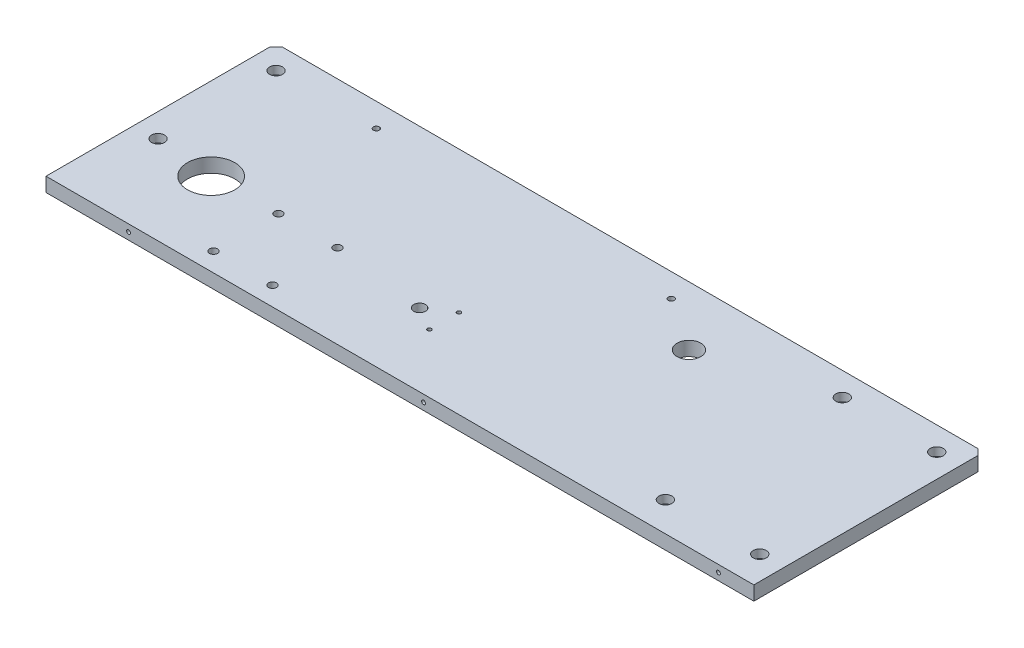
from build123d import *

# Parameters (mm, degrees)
SKETCH1_W                                         = 600
SKETCH1_H                                         = 195
EXTRUDE1_DEPTH                                    = 6
CHAMFER1_SIZE                                     = 5
M6_SOCKET_HEAD_CAP_SCREW_COUNTERBORE1_D           = 6.6
M6_SOCKET_HEAD_CAP_SCREW_COUNTERBORE1_CBORE_D     = 11
M6_SOCKET_HEAD_CAP_SCREW_COUNTERBORE1_CBORE_DEPTH = 7
M4_TAPPED_HOLE1_D                                 = 3.3
M4_TAPPED_HOLE1_DEPTH                             = 10.1
M4_TAPPED_HOLE1_TIP                               = 0.991420021
M8_TAPPED_HOLE1_D                                 = 6.8
M6_TAPPED_HOLE2_D                                 = 5
SKETCH10_R                                        = 20
CUT_EXTRUDE1_DEPTH                                = 316.674278331
SKETCH11_R                                        = 10
CUT_EXTRUDE2_DEPTH                                = 316.674278331
M4_TAPPED_HOLE2_D                                 = 3.3
M4_TAPPED_HOLE2_DEPTH                             = 12
M4_TAPPED_HOLE2_TIP                               = 0.991420021
SKETCH13_R                                        = 5
CUT_EXTRUDE3_DEPTH                                = 316.674278331


with BuildPart() as part:
    # Sketch1 → Extrude1 (new, symmetric)
    with BuildSketch(Plane(origin=(0, 0, 0), x_dir=(1, 0, 0), z_dir=(0, 1, 0))):
        Rectangle(SKETCH1_W, SKETCH1_H)
    extrude(amount=EXTRUDE1_DEPTH, both=True)

    # Chamfer1
    chamfer1_edges = [part.edges().sort_by_distance(p)[0] for p in [
        (-300, 0, -97.5),
        (300, 0, -97.5),
    ]]
    chamfer(chamfer1_edges, length=CHAMFER1_SIZE)

    # M6 Socket Head Cap Screw Counterbore1 (through all)
    with Locations(Plane(origin=(-280, 6, -77.5), x_dir=(0, 0, 1), z_dir=(0, 1, 0))):
        with Locations((0, 0), (100, 0), (0, 480), (0, 560), (150, 560), (150, 480)):
            CounterBoreHole(M6_SOCKET_HEAD_CAP_SCREW_COUNTERBORE1_D / 2, M6_SOCKET_HEAD_CAP_SCREW_COUNTERBORE1_CBORE_D / 2, M6_SOCKET_HEAD_CAP_SCREW_COUNTERBORE1_CBORE_DEPTH)

    # M4 Tapped Hole1
    with Locations(Plane(origin=(-230, 0, 97.5), x_dir=(1, 0, 0), z_dir=(0, 0, 1))):
        with Locations((0, 0), (250, 0), (500, 0)):
            Hole(M4_TAPPED_HOLE1_D / 2, depth=M4_TAPPED_HOLE1_DEPTH)
            with Locations((0, 0, -(M4_TAPPED_HOLE1_DEPTH + M4_TAPPED_HOLE1_TIP / 2))):  # 118° drill point
                Cone(0, M4_TAPPED_HOLE1_D / 2, M4_TAPPED_HOLE1_TIP, mode=Mode.SUBTRACT)

    # M8 Tapped Hole1 (through all)
    with Locations(Plane(origin=(-174, 6, 81.5), x_dir=(0, 0, 1), z_dir=(0, 1, 0))):
        with Locations((0, 0), (0, 50), (-55, 50), (-55, 0)):
            Hole(M8_TAPPED_HOLE1_D / 2)

    # M6 Tapped Hole2 (through all)
    with Locations(Plane(origin=(55, 6, -77.5), x_dir=(0, 0, 1), z_dir=(0, 1, 0))):
        with Locations((0, 0), (0, -250)):
            Hole(M6_TAPPED_HOLE2_D / 2)

    # Sketch10 → Cut-Extrude1 (cut, through all)
    with BuildSketch(Plane(origin=(0, 6, 0), x_dir=(1, 0, 0), z_dir=(0, 1, 0))):
        with Locations(Location((-230, -27.5, 0), (0, 0, 270))):
            Circle(SKETCH10_R)
    extrude(amount=-CUT_EXTRUDE1_DEPTH, mode=Mode.SUBTRACT)

    # Sketch11 → Cut-Extrude2 (cut, through all)
    with BuildSketch(Plane(origin=(0, 6, 0), x_dir=(1, 0, 0), z_dir=(0, 1, 0))):
        with Locations(Location((100, 47.5, 0), (0, 0, 270))):
            Circle(SKETCH11_R)
    extrude(amount=-CUT_EXTRUDE2_DEPTH, mode=Mode.SUBTRACT)

    # M4 Tapped Hole2
    with Locations(Plane(origin=(-25, 6, 47.5), x_dir=(0, 0, 1), z_dir=(0, 1, 0))):
        with Locations((0, 0), (-25, 0)):
            Hole(M4_TAPPED_HOLE2_D / 2, depth=M4_TAPPED_HOLE2_DEPTH)
            with Locations((0, 0, -(M4_TAPPED_HOLE2_DEPTH + M4_TAPPED_HOLE2_TIP / 2))):  # 118° drill point
                Cone(0, M4_TAPPED_HOLE2_D / 2, M4_TAPPED_HOLE2_TIP, mode=Mode.SUBTRACT)

    # Sketch13 → Cut-Extrude3 (cut, through all)
    with BuildSketch(Plane(origin=(0, 6, 0), x_dir=(1, 0, 0), z_dir=(0, 1, 0))):
        with Locations(Location((-45, -35.825, 0), (0, 0, 270))):
            Circle(SKETCH13_R)
    extrude(amount=-CUT_EXTRUDE3_DEPTH, mode=Mode.SUBTRACT)


solid = part.part
